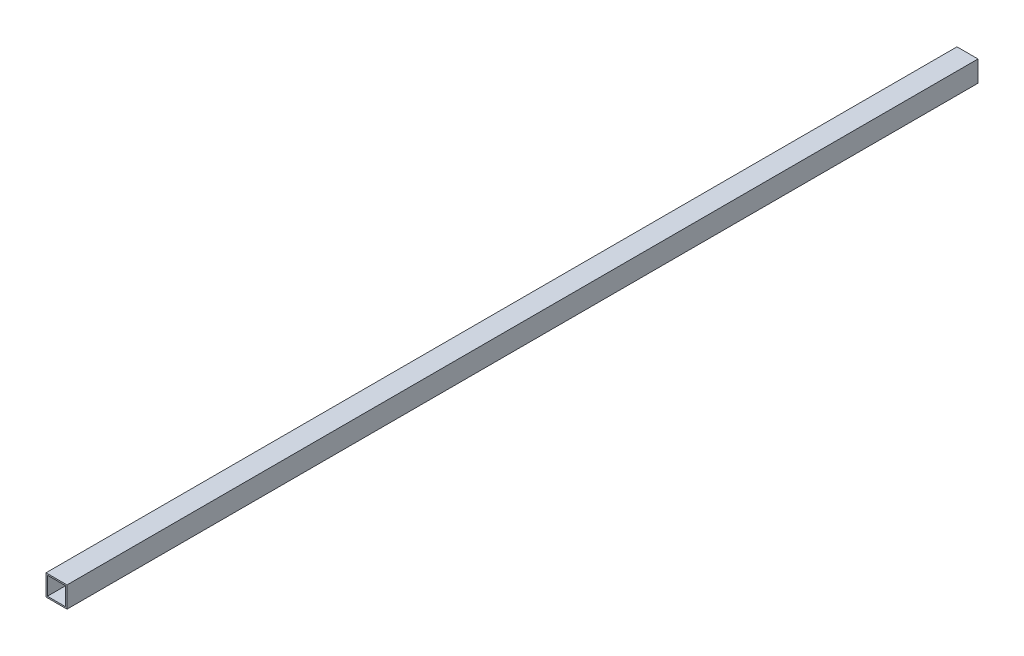
SolidWorks part; units mm, degrees
ref_plane "前视基准面" through (0, 0, 0) normal (0, 0, 1) x (1, 0, 0)
ref_plane "上视基准面" through (0, 0, 0) normal (0, 1, 0) x (1, 0, 0)
ref_plane "右视基准面" through (0, 0, 0) normal (1, 0, 0) x (0, 0, -1)
sketch "草图1" plane through (0, 0, 0) normal (0, 0, 1) x (1, 0, 0)
  line L0 (13, -13) -> (13, 13)
  line L1 (15, -15) -> (-15, -15)
  line L2 (15, -15) -> (15, 15)
  line L3 (15, 15) -> (-15, 15)
  line L4 (-15, -15) -> (-15, 15)
  line L5 (15, -15) -> (-15, 15) construction
  line L6 (15, 15) -> (-15, -15) construction
  line L7 (13, 13) -> (-13, 13)
  line L8 (-13, -13) -> (-13, 13)
  line L9 (13, -13) -> (-13, -13)
  point P0 (0, 0)
  dimension "D1" = 30
  dimension "D2" = 2
extrude "凸台-拉伸1" add sketch "草图1" along normal mid plane 1300
sketch "草图2" plane through (0, 0, 650) normal (0, 0, 1) x (1, 0, 0)
  circle A1 centre (0, 0) radius 4.2683
